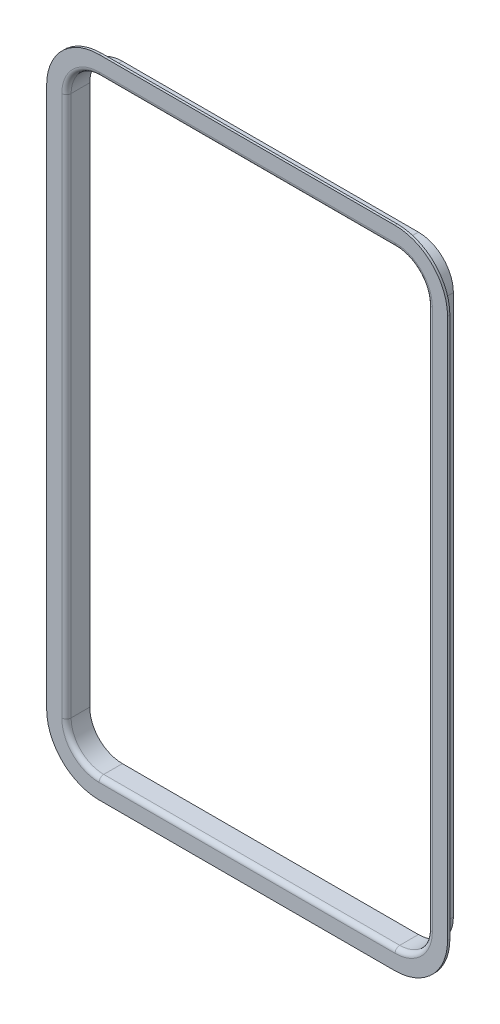
SolidWorks part; units mm, degrees
material "1023 碳钢板 (SS)"
ref_plane "Front Plane" through (0, 0, 0) normal (0, 0, 1) x (1, 0, 0)
ref_plane "Top Plane" through (0, 0, 0) normal (0, 1, 0) x (1, 0, 0)
ref_plane "Right Plane" through (0, 0, 0) normal (1, 0, 0) x (0, 0, -1)
sketch "Sketch1" plane through (0, 0, 0) normal (0, 0, 1) x (1, 0, 0)
  line L1 (-127, 260) -> (127, 260)
  line L2 (-155, 232) -> (-155, -232)
  line L3 (-127, -260) -> (127, -260)
  line L4 (155, 232) -> (155, -232)
  line L5 (-155, 260) -> (155, -260) construction
  line L6 (-155, -260) -> (155, 260) construction
  arc A0 (-155, -232) -> (-127, -260) centre (-127, -232) ccw
  arc A1 (155, -232) -> (127, -260) centre (127, -232) cw
  arc A2 (127, 260) -> (155, 232) centre (127, 232) cw
  arc A3 (-127, 260) -> (-155, 232) centre (-127, 232) ccw
  point P0 (0, 0)
  dimension "D3" = 28
  dimension "D4" = 28
  dimension "D5" = 28
  dimension "D6" = 28
  dimension "D1" = 520
  dimension "D2" = 310
sketch "Sketch2" plane through (0, 0, 0) normal (0, 1, 0) x (1, 0, 0)
  line L0 (155, 4) -> (155, 20)
  line L1 (-155, 0) -> (155, 0) construction
  line L2 (-155, 0) -> (155, 0) construction
  line L3 (155, 20) -> (157, 20)
  line L4 (157, 20) -> (157, 4)
  line L5 (159, 2) -> (172, 2)
  line L6 (172, 2) -> (172, 0)
  line L7 (172, 0) -> (159, 0)
  line L8 (155, 10.8048) -> (155, -12.1668) construction
  arc A0 (157, 4) -> (159, 2) centre (159, 4) ccw
  arc A1 (155, 4) -> (159, 0) centre (159, 4) ccw
  point P12 (157, 2)
  point P15 (155, 0)
  dimension "D5" = 2
  dimension "D6" = 4
  dimension "D1" = 20
  dimension "D2" = 15
  dimension "D3" = 2
  dimension "D4" = 2
  dimension "D7" = 155
sweep "Sweep1" add profiles "Sketch2" path "Sketch1"
